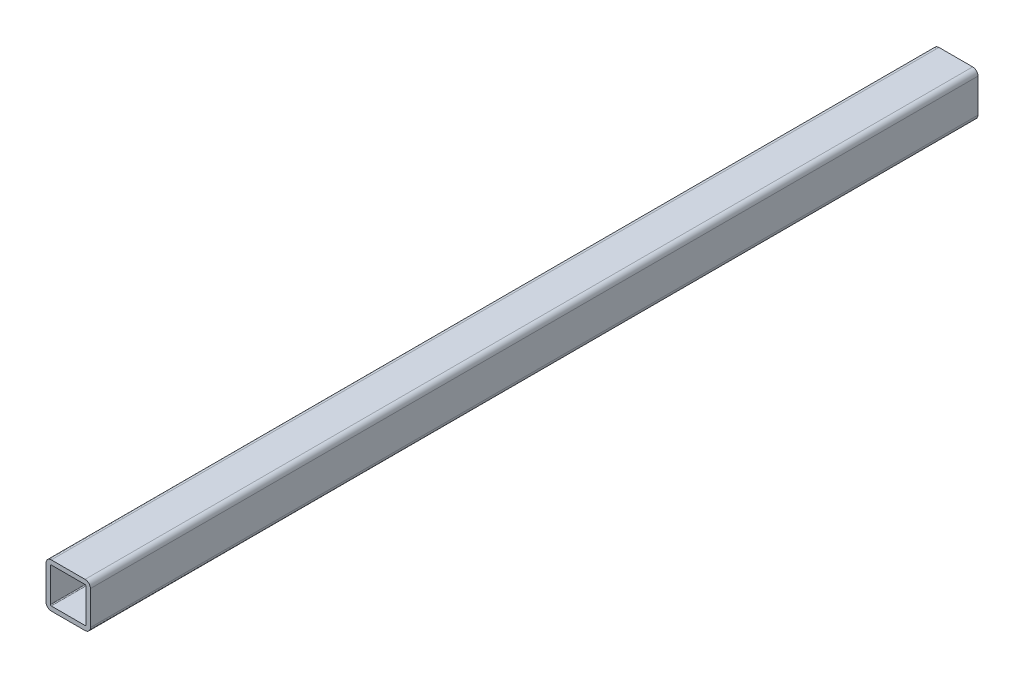
SolidWorks part; units mm, degrees
material "Q235B"
ref_plane "Front Plane" through (0, 0, 0) normal (0, 0, 1) x (1, 0, 0)
ref_plane "Top Plane" through (0, 0, 0) normal (0, 1, 0) x (1, 0, 0)
ref_plane "Right Plane" through (0, 0, 0) normal (1, 0, 0) x (0, 0, -1)
sketch "Sketch1" plane through (0, 0, 0) normal (0, 0, 1) x (1, 0, 0)
  line L0 (6, 45) -> (44, 45)
  line L1 (6, 0) -> (44, 0)
  line L2 (0, 6) -> (0, 44)
  line L3 (6, 50) -> (44, 50)
  line L4 (50, 6) -> (50, 44)
  line L5 (45, 6) -> (45, 44)
  line L6 (6, 5) -> (44, 5)
  line L7 (5, 6) -> (5, 44)
  arc A0 (6, 0) -> (0, 6) centre (6, 6) cw
  arc A1 (44, 0) -> (50, 6) centre (44, 6) ccw
  arc A2 (44, 50) -> (50, 44) centre (44, 44) cw
  arc A3 (0, 44) -> (6, 50) centre (6, 44) cw
  arc A4 (5, 44) -> (6, 45) centre (6, 44) cw
  arc A5 (44, 45) -> (45, 44) centre (44, 44) cw
  arc A6 (44, 5) -> (45, 6) centre (44, 6) ccw
  arc A7 (6, 5) -> (5, 6) centre (6, 6) cw
  point P7 (0, 0)
  point P12 (50, 50)
  point P15 (0, 50)
  dimension "D3" = 6
  dimension "D1" = 50
  dimension "D2" = 50
  dimension "D4" = 5
extrude "Boss-Extrude1" add sketch "Sketch1" along normal blind 1000
